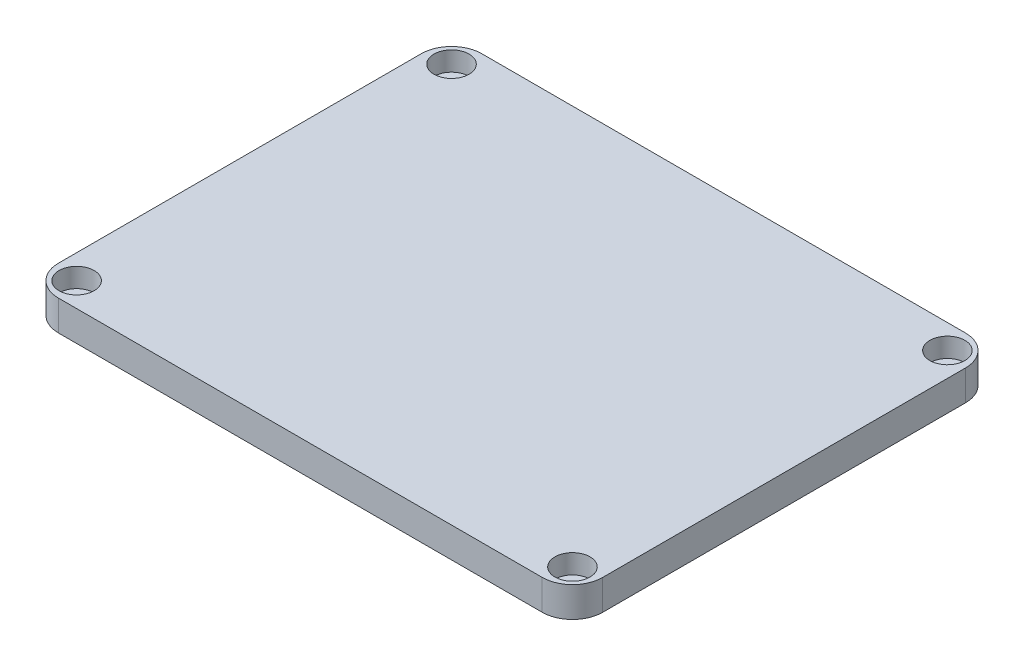
SolidWorks part; units mm, degrees
ref_plane "Front Plane" through (0, 0, 0) normal (0, 0, 1) x (1, 0, 0)
ref_plane "Top Plane" through (0, 0, 0) normal (0, 1, 0) x (1, 0, 0)
ref_plane "Right Plane" through (0, 0, 0) normal (1, 0, 0) x (0, 0, -1)
sketch "Sketch1" plane through (0, 0, 0) normal (0, 1, 0) x (1, 0, 0)
  line L1 (-40, -35) -> (40, -35)
  line L2 (-45, -30) -> (-45, 30)
  line L3 (-40, 35) -> (40, 35)
  line L4 (45, -30) -> (45, 30)
  line L5 (-45, -35) -> (45, 35) construction
  line L6 (-45, 35) -> (45, -35) construction
  arc A0 (-40, -35) -> (-45, -30) centre (-40, -30) cw
  arc A1 (40, -35) -> (45, -30) centre (40, -30) ccw
  arc A2 (40, 35) -> (45, 30) centre (40, 30) cw
  arc A3 (-45, 30) -> (-40, 35) centre (-40, 30) cw
  circle A4 centre (-41, 31) radius 1.6
  circle A5 centre (-41, -31) radius 1.6
  circle A6 centre (41, -31) radius 1.6
  circle A7 centre (41, 31) radius 1.6
  point P0 (0, 0)
  dimension "D3" = 5
  dimension "D4" = 3.2
  dimension "D5" = 4
  dimension "D6" = 4
  dimension "D7" = 4
  dimension "D8" = 4
  dimension "D9" = 4
  dimension "D10" = 4
  dimension "D11" = 4
  dimension "D12" = 4
  dimension "D1" = 90
  dimension "D2" = 70
extrude "Boss-Extrude1" add sketch "Sketch1" along normal blind 5
sketch "Sketch2" plane through (0, 5, 0) normal (0, 1, 0) x (1, 0, 0)
  circle A0 centre (41, 31) radius 2.9
  circle A1 centre (-41, 31) radius 2.9
  circle A2 centre (-41, -31) radius 2.9
  circle A3 centre (41, -31) radius 2.9
  dimension "D1" = 5.8
extrude "Cut-Extrude1" cut sketch "Sketch2" against normal blind 3.2
